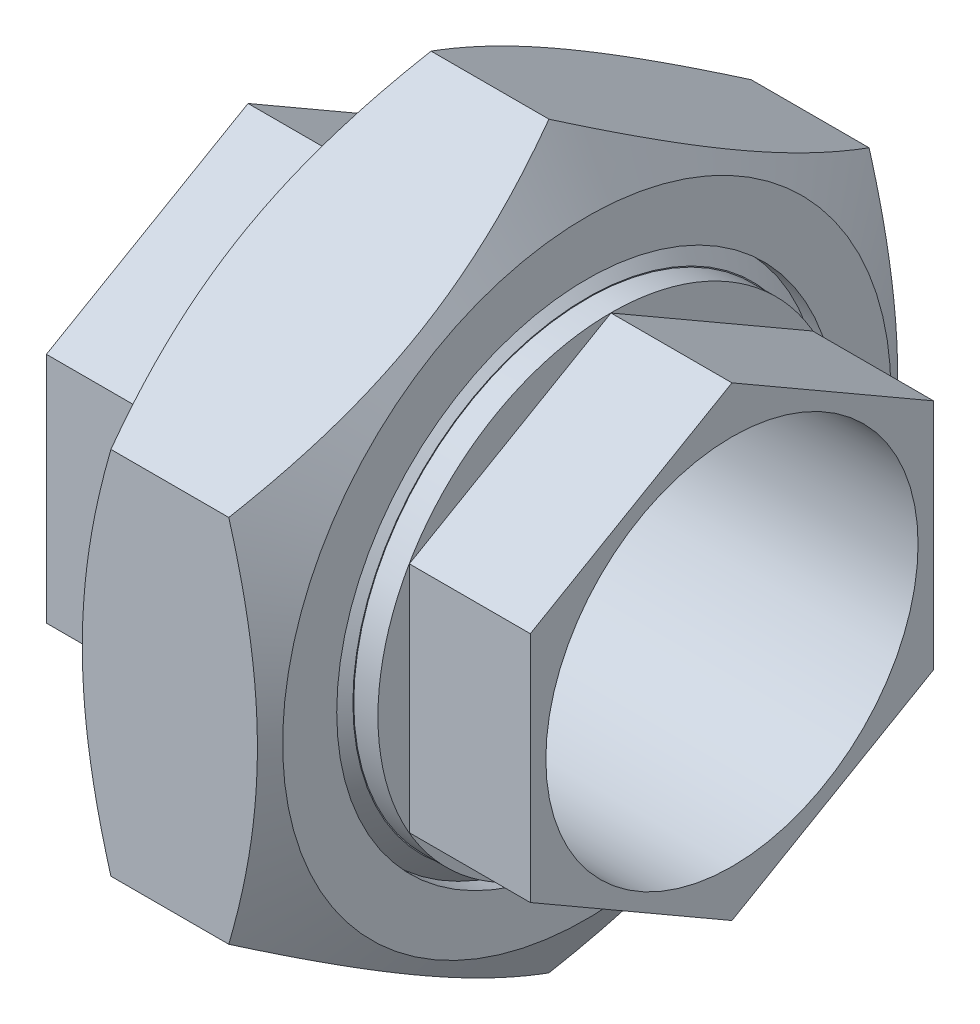
SolidWorks part; units mm, degrees
material "黑心可锻铸铁-KTH350-10"
ref_plane "前视基准面" through (0, 0, 0) normal (0, 0, 1) x (1, 0, 0)
ref_plane "上视基准面" through (0, 0, 0) normal (0, 1, 0) x (1, 0, 0)
ref_plane "右视基准面" through (0, 0, 0) normal (1, 0, 0) x (0, 0, -1)
sketch "草图1" plane through (0, 0, 0) normal (0, 0, 1) x (1, 0, 0)
  line L0 (0, 0) -> (0, 40.3075) construction
  line L1 (0, 0) -> (39, 0) construction
  line L2 (39, 35.05) -> (15.6, 35.05)
  line L3 (15.6, 35.05) -> (15.6, 40.3075)
  line L4 (15.6, 40.3075) -> (0, 40.3075)
  line L5 (0, 40.3075) -> (0, 46.266)
  line L6 (0, 46.266) -> (-15.6, 46.266)
  line L7 (-15.6, 46.266) -> (-15.6, 35.05)
  line L8 (-15.6, 35.05) -> (-39, 35.05)
  line L9 (-39, 35.05) -> (-39, 26.8771)
  line L10 (-39, 26.8771) -> (-15.6, 26.06)
  line L11 (-15.6, 26.06) -> (15.6, 26.06)
  line L12 (15.6, 26.06) -> (39, 26.8771)
  line L13 (39, 26.8771) -> (39, 35.05)
  line L14 (-15.6, 46.266) -> (-15.6, 59.585) construction
  line L15 (-15.6, 59.585) -> (15.6, 59.585) construction
  line L16 (15.6, 59.585) -> (15.6, 40.3075) construction
revolve "旋转1" add sketch "草图1" angle 360 about L1
chamfer "倒角1" distance 2.606 angle 45 2 edges at (-15.6, 0, 46.266) (15.6, 0, 40.3075)
sketch "草图3" plane through (0, 0, 0) normal (0, 0, 1) x (1, 0, 0)
  line L0 (-15.6, 46.266) -> (-15.6, 59.585)
  line L1 (-15.6, 59.585) -> (15.6, 59.585)
  line L2 (15.6, 59.585) -> (15.6, 40.3075)
  line L3 (15.6, 40.3075) -> (0, 40.3075)
  line L4 (0, 40.3075) -> (0, 46.266)
  line L5 (0, 46.266) -> (-15.6, 46.266)
  line L6 (0, 0) -> (14.2687, 0) construction
  line L7 (0, 0) -> (39, 0) construction
revolve "旋转2" add sketch "草图3" angle 360 about L6
sketch "草图4" plane through (39, 0, 0) normal (1, 0, 0) x (0, 0, -1)
  line L1 (0, 35.05) -> (-30.3542, 17.525)
  line L2 (-30.3542, 17.525) -> (-30.3542, -17.525)
  line L3 (-30.3542, -17.525) -> (0, -35.05)
  line L4 (0, -35.05) -> (30.3542, -17.525)
  line L5 (30.3542, -17.525) -> (30.3542, 17.525)
  line L6 (30.3542, 17.525) -> (0, 35.05)
  circle A0 centre (0, 0) radius 30.3542 construction
  circle A2 centre (0, 0) radius 35.05 construction
  circle A3 centre (0, 0) radius 40.3075 construction
  circle A4 centre (0, 0) radius 40.3075
  dimension "D1" = 60.7084
extrude "切除-拉伸1" cut sketch "草图4" against normal blind 19.5
sketch "草图5" plane through (39, 0, 0) normal (1, 0, 0) x (0, 0, -1)
  circle A0 centre (0, 0) radius 28.3905
sketch "草图6" plane through (0, 0, 0) normal (0, 0, 1) x (1, 0, 0)
  line L0 (15.6, 35.05) -> (15.6, 40.3075) construction
  line L1 (15.6, -59.585) -> (15.6, 59.585) construction
  line L2 (25.472, 26.4047) -> (15.6, 26.4047)
  line L3 (15.6, 26.4047) -> (15.6, 36.2767)
  line L4 (0, 0) -> (39, 0) construction
  line L5 (39, 26.8771) -> (15.6, 26.06) construction
  arc A0 (15.6, 36.2767) -> (25.472, 26.4047) centre (25.472, 36.2767) ccw
revolve "旋转3" add sketch "草图6" angle 360 about L4
sketch "草图8" plane through (15.6, 0, 0) normal (1, 0, 0) x (0, 0, -1)
  line L1 (0, 59.585) -> (-51.6021, 29.7925)
  line L2 (-51.6021, 29.7925) -> (-51.6021, -29.7925)
  line L3 (-51.6021, -29.7925) -> (0, -59.585)
  line L4 (0, -59.585) -> (51.6021, -29.7925)
  line L5 (51.6021, -29.7925) -> (51.6021, 29.7925)
  line L6 (51.6021, 29.7925) -> (0, 59.585)
  circle A0 centre (0, 0) radius 51.6021 construction
  circle A1 centre (0, 0) radius 59.585 construction
  circle A2 centre (0, 0) radius 65.5435
extrude "切除-拉伸3" cut sketch "草图8" against normal through all
sketch "草图10" plane through (15.6, 0, 0) normal (1, 0, 0) x (0, 0, -1)
  circle A0 centre (0, 0) radius 49.022
extrude "切除-拉伸4" cut sketch "草图10" against normal blind 10 draft 60 flip side to cut
mirror "镜向7" about plane through (0, 0, 0) normal (1, 0, 0) of "切除-拉伸4", "切除-拉伸1", "旋转3"
sketch "草图11" plane through (-39, 0, 0) normal (-1, 0, 0) x (0, 0, 1)
  circle A0 centre (0, 0) radius 30
  dimension "D1" = 60
extrude "切除-拉伸5" cut sketch "草图11" against normal through all
sketch "草图12" plane through (-39, 0, 0) normal (-1, 0, 0) x (0, 0, 1)
  line L1 (0, 37.5278) -> (-32.5, 18.7639)
  line L2 (-32.5, 18.7639) -> (-32.5, -18.7639)
  line L3 (-32.5, -18.7639) -> (0, -37.5278)
  line L4 (0, -37.5278) -> (32.5, -18.7639)
  line L5 (32.5, -18.7639) -> (32.5, 18.7639)
  line L6 (32.5, 18.7639) -> (0, 37.5278)
  circle A0 centre (0, 0) radius 32.5 construction
  circle A1 centre (0, 0) radius 30
  dimension "D1" = 65
extrude "凸台-拉伸1" add sketch "草图12" against normal up to surface (19.5 mm away) up to face at (-19.5, 28.3208, -16.351)
sketch "草图13" plane through (-19.5, 0, 0) normal (-1, 0, 0) x (0, 0, 1)
  circle A0 centre (0, 0) radius 35.05
  circle A1 centre (0, 0) radius 37.5589
extrude "凸台-拉伸2" add sketch "草图13" against normal up to surface (35.1 mm away)
ref_plane "基准面1" through (0, 0, 0) normal (1, 0, 0) x (0, 0, -1)
mirror "镜向8" about plane through (0, 0, 0) normal (1, 0, 0) of "凸台-拉伸2", "凸台-拉伸1"
equation "\"D3@草图1\" = \"L@草图1\" * 0.4"
equation "\"D4@草图1\" = \"D@草图1\"*1.15"
equation "\"D5@草图1\" = \"D@草图1\"*1.32"
equation "\"D6@草图1\" = \"D@草图1\"*1.7"
equation "\"D1@草图5\" = \"D@草图1\" * 0.81"
equation "\"D1@切除-拉伸1\" = \"L@草图1\"*0.25"
equation "\"D1@草图6\" = \"D4@草图1\"*0.9"
equation "\"D1@草图8\" = \"D6@草图1\" * 1.1"
equation "\"D1@草图10\" = \"D2@草图8\"*0.95"
